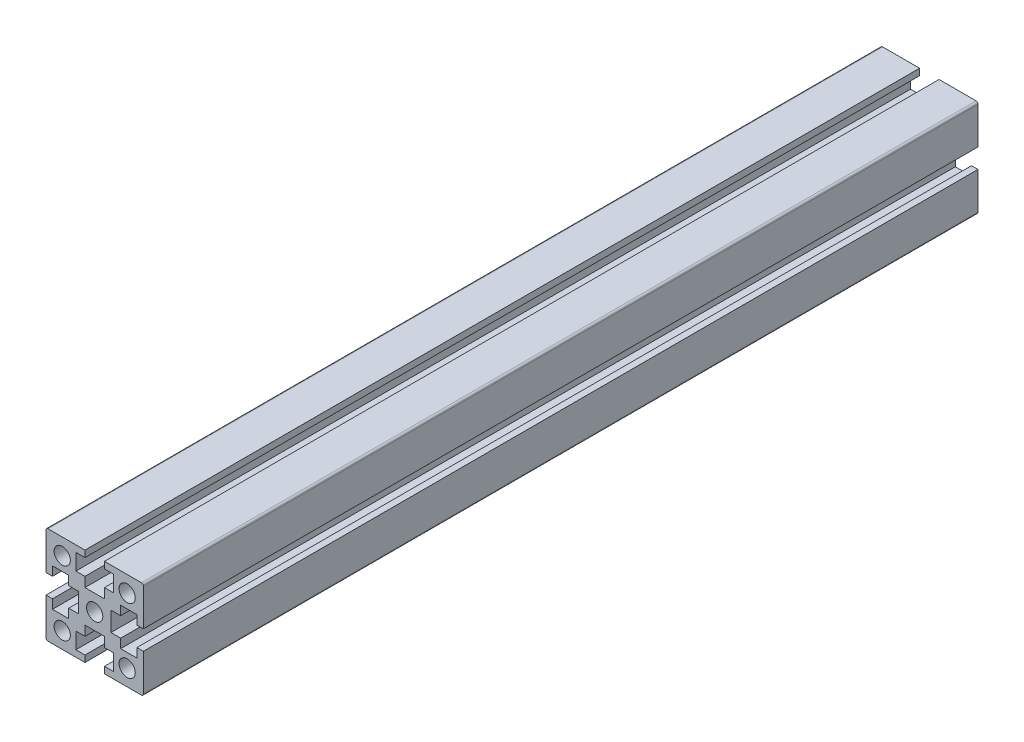
from build123d import *

# Parameters (mm, degrees)
SKETCH4_R           = 1.25
BOSS_EXTRUDE3_DEPTH = 100
SCALE_1_SCALE       = 0.7
SKETCH5_R           = 0.875
BOSS_EXTRUDE4_DEPTH = 20


with BuildPart() as part:
    # Sketch4 → Boss-Extrude3 (new body)
    with BuildSketch(Plane.XY):
        with BuildLine():
            Line((-1.5, 7.5), (-7.2, 7.5))
            ThreePointArc((-7.2, 7.5), (-7.412132034, 7.412132034), (-7.5, 7.2))
            Line((-7.5, 7.2), (-7.5, 1.5))
            Line((-7.5, 1.5), (-6.5, 1.5))
            Line((-6.5, 1.5), (-6.5, 2.9))
            Line((-6.5, 2.9), (-4, 2.9))
            Line((-4, 2.9), (-4, 1.5))
            Line((-4, 1.5), (-2.5, 1.5))
            Line((-2.5, 1.5), (-2.5, -1.5))
            Line((-2.5, -1.5), (-4, -1.5))
            Line((-4, -1.5), (-4, -2.9))
            Line((-4, -2.9), (-6.5, -2.9))
            Line((-6.5, -2.9), (-6.5, -1.5))
            Line((-6.5, -1.5), (-7.5, -1.5))
            Line((-7.5, -1.5), (-7.5, -7.2))
            ThreePointArc((-7.5, -7.2), (-7.412132034, -7.412132034), (-7.2, -7.5))
            Line((-7.2, -7.5), (-1.5, -7.5))
            Line((-1.5, -7.5), (-1.5, -6.5))
            Line((-1.5, -6.5), (-2.9, -6.5))
            Line((-2.9, -6.5), (-2.9, -4))
            Line((-2.9, -4), (-1.5, -4))
            Line((-1.5, -4), (-1.5, -2.5))
            Line((-1.5, -2.5), (1.5, -2.5))
            Line((1.5, -2.5), (1.5, -4))
            Line((1.5, -4), (2.9, -4))
            Line((2.9, -4), (2.9, -6.5))
            Line((2.9, -6.5), (1.5, -6.5))
            Line((1.5, -6.5), (1.5, -7.5))
            Line((1.5, -7.5), (7.2, -7.5))
            ThreePointArc((7.2, -7.5), (7.412132034, -7.412132034), (7.5, -7.2))
            Line((7.5, -7.2), (7.5, -1.5))
            Line((7.5, -1.5), (6.5, -1.5))
            Line((6.5, -1.5), (6.5, -2.9))
            Line((6.5, -2.9), (4, -2.9))
            Line((4, -2.9), (4, -1.5))
            Line((4, -1.5), (2.5, -1.5))
            Line((2.5, -1.5), (2.5, 1.5))
            Line((2.5, 1.5), (4, 1.5))
            Line((4, 1.5), (4, 2.9))
            Line((4, 2.9), (6.5, 2.9))
            Line((6.5, 2.9), (6.5, 1.5))
            Line((6.5, 1.5), (7.5, 1.5))
            Line((7.5, 1.5), (7.5, 7.2))
            ThreePointArc((7.5, 7.2), (7.412132034, 7.412132034), (7.2, 7.5))
            Line((7.2, 7.5), (1.5, 7.5))
            Line((1.5, 7.5), (1.5, 6.5))
            Line((1.5, 6.5), (2.9, 6.5))
            Line((2.9, 6.5), (2.9, 4))
            Line((2.9, 4), (1.5, 4))
            Line((1.5, 4), (1.5, 2.5))
            Line((1.5, 2.5), (-1.5, 2.5))
            Line((-1.5, 2.5), (-1.5, 4))
            Line((-1.5, 4), (-2.9, 4))
            Line((-2.9, 4), (-2.9, 6.5))
            Line((-2.9, 6.5), (-1.5, 6.5))
            Line((-1.5, 6.5), (-1.5, 7.5))
        make_face()
        with Locations((-5, -5)):
            Circle(SKETCH4_R, mode=Mode.SUBTRACT)
        Circle(SKETCH4_R, mode=Mode.SUBTRACT)
        with Locations((5, -5)):
            Circle(SKETCH4_R, mode=Mode.SUBTRACT)
        with Locations((-5, 5)):
            Circle(SKETCH4_R, mode=Mode.SUBTRACT)
        with Locations((5, 5)):
            Circle(SKETCH4_R, mode=Mode.SUBTRACT)
    extrude(amount=BOSS_EXTRUDE3_DEPTH)


with BuildPart() as part_1:
    # Scale 1: scaled about (0, 0, 0)
    add(part.part.scale(SCALE_1_SCALE))

    # Sketch5 → Boss-Extrude4 (add)
    with BuildSketch(Plane.XY.offset(70)):
        with BuildLine():
            Line((-1.05, 5.25), (-5.04, 5.25))
            ThreePointArc((-5.04, 5.25), (-5.188492424, 5.188492424), (-5.25, 5.04))
            Line((-5.25, 5.04), (-5.25, 1.05))
            Line((-5.25, 1.05), (-4.55, 1.05))
            Line((-4.55, 1.05), (-4.55, 2.03))
            Line((-4.55, 2.03), (-2.8, 2.03))
            Line((-2.8, 2.03), (-2.8, 1.05))
            Line((-2.8, 1.05), (-1.75, 1.05))
            Line((-1.75, 1.05), (-1.75, -1.05))
            Line((-1.75, -1.05), (-2.8, -1.05))
            Line((-2.8, -1.05), (-2.8, -2.03))
            Line((-2.8, -2.03), (-4.55, -2.03))
            Line((-4.55, -2.03), (-4.55, -1.05))
            Line((-4.55, -1.05), (-5.25, -1.05))
            Line((-5.25, -1.05), (-5.25, -5.04))
            ThreePointArc((-5.25, -5.04), (-5.188492424, -5.188492424), (-5.04, -5.25))
            Line((-5.04, -5.25), (-1.05, -5.25))
            Line((-1.05, -5.25), (-1.05, -4.55))
            Line((-1.05, -4.55), (-2.03, -4.55))
            Line((-2.03, -4.55), (-2.03, -2.8))
            Line((-2.03, -2.8), (-1.05, -2.8))
            Line((-1.05, -2.8), (-1.05, -1.75))
            Line((-1.05, -1.75), (1.05, -1.75))
            Line((1.05, -1.75), (1.05, -2.8))
            Line((1.05, -2.8), (2.03, -2.8))
            Line((2.03, -2.8), (2.03, -4.55))
            Line((2.03, -4.55), (1.05, -4.55))
            Line((1.05, -4.55), (1.05, -5.25))
            Line((1.05, -5.25), (5.04, -5.25))
            ThreePointArc((5.04, -5.25), (5.188492424, -5.188492424), (5.25, -5.04))
            Line((5.25, -5.04), (5.25, -1.05))
            Line((5.25, -1.05), (4.55, -1.05))
            Line((4.55, -1.05), (4.55, -2.03))
            Line((4.55, -2.03), (2.8, -2.03))
            Line((2.8, -2.03), (2.8, -1.05))
            Line((2.8, -1.05), (1.75, -1.05))
            Line((1.75, -1.05), (1.75, 1.05))
            Line((1.75, 1.05), (2.8, 1.05))
            Line((2.8, 1.05), (2.8, 2.03))
            Line((2.8, 2.03), (4.55, 2.03))
            Line((4.55, 2.03), (4.55, 1.05))
            Line((4.55, 1.05), (5.25, 1.05))
            Line((5.25, 1.05), (5.25, 5.04))
            ThreePointArc((5.25, 5.04), (5.188492424, 5.188492424), (5.04, 5.25))
            Line((5.04, 5.25), (1.05, 5.25))
            Line((1.05, 5.25), (1.05, 4.55))
            Line((1.05, 4.55), (2.03, 4.55))
            Line((2.03, 4.55), (2.03, 2.8))
            Line((2.03, 2.8), (1.05, 2.8))
            Line((1.05, 2.8), (1.05, 1.75))
            Line((1.05, 1.75), (-1.05, 1.75))
            Line((-1.05, 1.75), (-1.05, 2.8))
            Line((-1.05, 2.8), (-2.03, 2.8))
            Line((-2.03, 2.8), (-2.03, 4.55))
            Line((-2.03, 4.55), (-1.05, 4.55))
            Line((-1.05, 4.55), (-1.05, 5.25))
        make_face()
        with Locations((3.5, -3.5)):
            Circle(SKETCH5_R, mode=Mode.SUBTRACT)
        with Locations((-3.5, -3.5)):
            Circle(SKETCH5_R, mode=Mode.SUBTRACT)
        with Locations((-3.5, 3.5)):
            Circle(SKETCH5_R, mode=Mode.SUBTRACT)
        with Locations((3.5, 3.5)):
            Circle(SKETCH5_R, mode=Mode.SUBTRACT)
        Circle(SKETCH5_R, mode=Mode.SUBTRACT)
    extrude(amount=BOSS_EXTRUDE4_DEPTH)


solid = part_1.part
